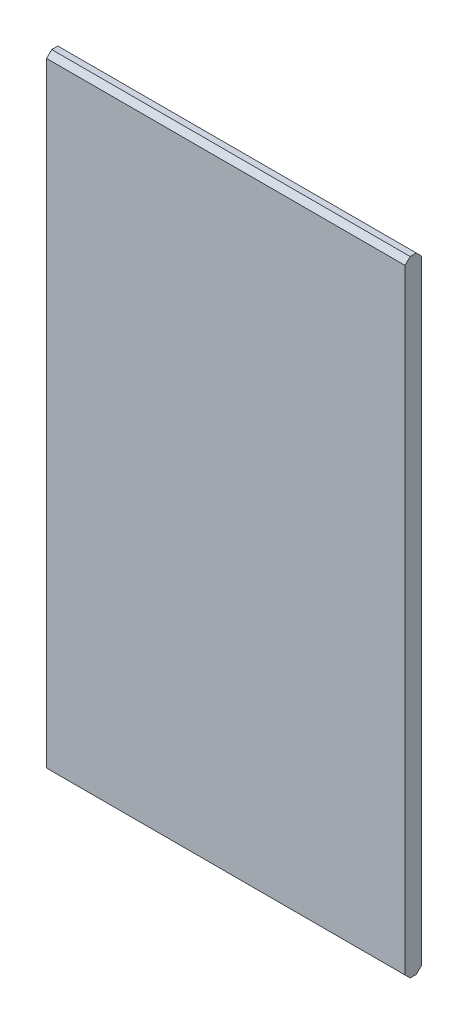
from build123d import *

# Parameters (mm, degrees)
SKETCH1_W           = 350
SKETCH1_H           = 610
BOSS_EXTRUDE1_DEPTH = 16
CHAMFER1_SIZE       = 5


with BuildPart() as part:
    # Sketch1 → Boss-Extrude1 (new body)
    with BuildSketch(Plane.XY):
        with Locations((175, 305)):
            Rectangle(SKETCH1_W, SKETCH1_H)
    extrude(amount=BOSS_EXTRUDE1_DEPTH)

    # Chamfer1
    chamfer1_edges = [part.edges().sort_by_distance(p)[0] for p in [
        (175, 610, 16),
        (175, 610, 0),
        (175, 0, 0),
        (175, 0, 16),
    ]]
    chamfer(chamfer1_edges, length=CHAMFER1_SIZE)


solid = part.part
